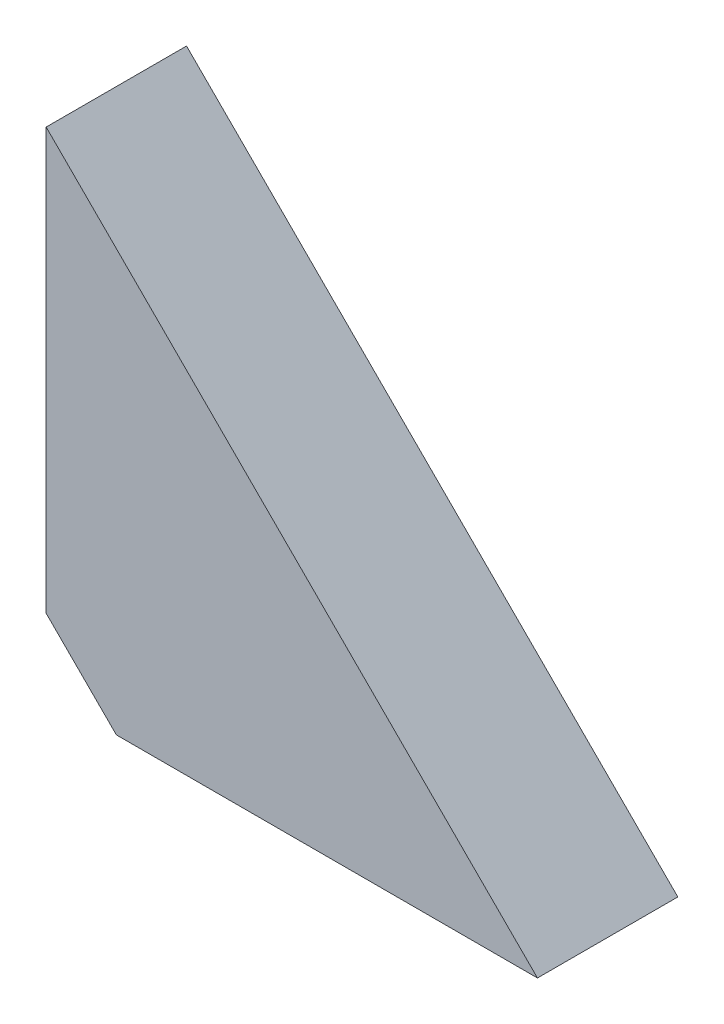
from build123d import *

# Parameters (mm, degrees)
EXTRUDE_1_DEPTH = 20
CHAMFER_1_SIZE  = 10


with BuildPart() as part:
    # 草图1 → 凸台-拉伸1 (new body)
    with BuildSketch(Plane.XY):
        Polygon((0, 70), (0, 0), (70, 0), align=None)
    extrude(amount=EXTRUDE_1_DEPTH)

    # 倒角1
    chamfer_1_edges = [part.edges().sort_by_distance(p)[0] for p in [
        (0, 0, 10),
    ]]
    chamfer(chamfer_1_edges, length=CHAMFER_1_SIZE)


solid = part.part
